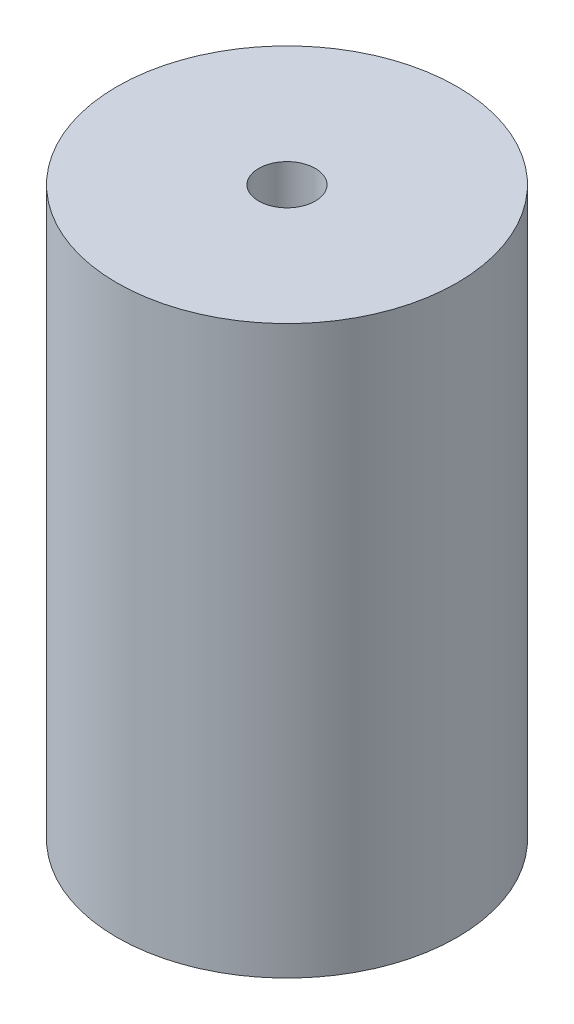
SolidWorks part; units mm, degrees
ref_plane "Front Plane" through (0, 0, 0) normal (0, 0, 1) x (1, 0, 0)
ref_plane "Top Plane" through (0, 0, 0) normal (0, 1, 0) x (1, 0, 0)
ref_plane "Right Plane" through (0, 0, 0) normal (1, 0, 0) x (0, 0, -1)
other "Configuration Table"
sketch "Sketch1" plane through (0, 0, 0) normal (0, 1, 0) x (1, 0, 0)
  circle A0 centre (0, 0) radius 60
  dimension "D1" = 120
extrude "Boss-Extrude2" add sketch "Sketch1" along normal blind 200
sketch "Sketch3" plane through (0, 200, 0) normal (0, 1, 0) x (1, 0, 0)
  circle A0 centre (0, 0) radius 10
  dimension "D1" = 20
extrude "Cut-Extrude2" cut sketch "Sketch3" against normal blind 40
cosmetic thread "Cosmetic Thread2"
